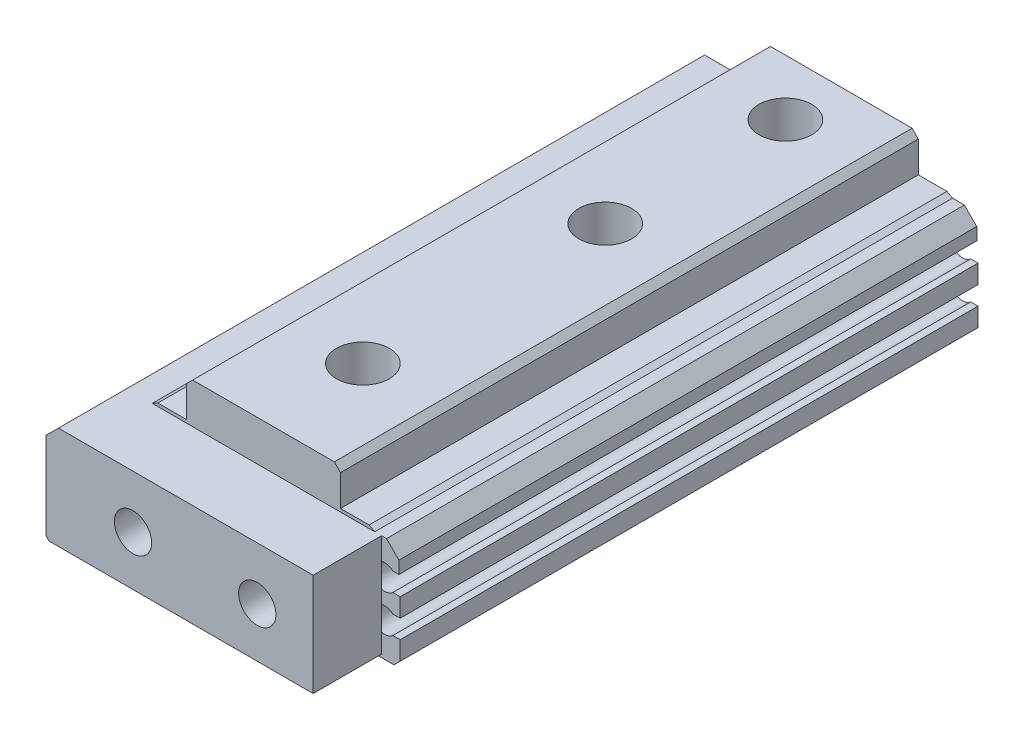
from build123d import *

# Parameters (mm, degrees)
EXTRUDE_1_DEPTH             = 93
EXTRUDE_2_DEPTH             = 11
CUT_EXTRUDE_1_DEPTH         = 93
PATTERN_LINEAR_1_COUNT      = 2
PATTERN_LINEAR_1_PITCH      = 6
CUT_EXTRUDE_2_DEPTH         = 93
CUT_EXTRUDE_3_DEPTH         = 93
PATTERN_LINEAR_2_COUNT      = 2
PATTERN_LINEAR_2_PITCH      = 8
PATTERN_LINEAR_2_COUNT_DIR2 = 2
PATTERN_LINEAR_2_PITCH_DIR2 = 20
PATTERN_LINEAR_3_COUNT      = 2
PATTERN_LINEAR_3_PITCH      = 20
CUT_EXTRUDE_4_DEPTH         = 4
PATTERN_LINEAR_4_COUNT      = 2
PATTERN_LINEAR_4_PITCH      = 58
SKETCH_16_W                 = 1
SKETCH_16_H                 = 9.5
CUT_EXTRUDE_5_DEPTH         = 46
SKETCH_21_W                 = 2
SKETCH_21_H                 = 4
CUT_EXTRUDE_6_DEPTH         = 93
PATTERN_LINEAR_5_COUNT      = 2
PATTERN_LINEAR_5_PITCH      = 8
HOLE_WIZARD_4_D             = 13
HOLE_WIZARD_4_DEPTH         = 1
HOLE_WIZARD_5_D             = 13
HOLE_WIZARD_5_DEPTH         = 1
HOLE_WIZARD_6_D             = 4.134
HOLE_WIZARD_6_DEPTH         = 5
HOLE_WIZARD_6_CSINK_D       = 5
HOLE_WIZARD_6_CSINK_ANGLE   = 90
HOLE_WIZARD_6_TIP           = 1.193383006


with BuildPart() as part:
    # 草图1 → 凸台-拉伸1 (new body)
    with BuildSketch(Plane.XY):
        Polygon((-24, 1.5), (-22.5, 0), (22, 0), (22, 17), (17.9, 17), (17, 17.5), (12.4, 17.5), (12.4, 22.5), (11.4, 23.5), (-11.4, 23.5), (-12.4, 22.5), (-12.4, 17.5), (-17, 17.5), (-17.9, 17), (-22, 17), (-24, 15), align=None)
    extrude(amount=EXTRUDE_1_DEPTH)

    # 草图2 → 凸台-拉伸2 (add)
    with BuildSketch(Plane.XY.offset(93)):
        Polygon((-24, 1), (-23.5, 0.5), (19, 0.5), (19, 17), (-22, 17), (-24, 15), align=None)
    extrude(amount=EXTRUDE_2_DEPTH)

    # 草图3 → 切除-拉伸1 (cut)
    with BuildSketch(Plane.XY):
        with BuildLine():
            Line((20.822875656, 4), (22, 4))
            Line((22, 4), (22, 7))
            Line((22, 7), (20.822875656, 7))
            ThreePointArc((20.822875656, 7), (17.5, 5.5), (20.822875656, 4))
        make_face()
    cut_extrude_1 = extrude(amount=CUT_EXTRUDE_1_DEPTH, mode=Mode.SUBTRACT)

    # 阵列(线性)1: 切除-拉伸1 ×2
    with Locations(*[(0, i * PATTERN_LINEAR_1_PITCH, 0) for i in range(1, PATTERN_LINEAR_1_COUNT)]):
        add(cut_extrude_1, mode=Mode.SUBTRACT)

    # 草图5 → 切除-拉伸2 (cut)
    with BuildSketch(Plane.XY):
        with BuildLine():
            Line((4.7, 0), (16, 0))
            Line((16, 0), (14.927664784, 1.072335216))
            ThreePointArc((14.927664784, 1.072335216), (14.37434682, 1.353332174), (13.761801698, 1.253790561))
            ThreePointArc((13.761801698, 1.253790561), (10.233759649, 0.343332602), (6.659563577, 1.051242793))
            ThreePointArc((6.659563577, 1.051242793), (6.070298822, 1.121297778), (5.5450865, 0.8450865))
            Line((5.5450865, 0.8450865), (4.7, 0))
        make_face()
    extrude(amount=CUT_EXTRUDE_2_DEPTH, mode=Mode.SUBTRACT)

    # 草图6 → 切除-拉伸3 (cut)
    with BuildSketch(Plane.XY):
        with BuildLine():
            Line((-16, 0), (-4.7, 0))
            Line((-4.7, 0), (-5.5450865, 0.8450865))
            ThreePointArc((-5.5450865, 0.8450865), (-6.070298822, 1.121297778), (-6.659563577, 1.051242793))
            ThreePointArc((-6.659563577, 1.051242793), (-10.233759649, 0.343332602), (-13.761801698, 1.253790561))
            ThreePointArc((-13.761801698, 1.253790561), (-14.37434682, 1.353332174), (-14.927664784, 1.072335216))
            Line((-14.927664784, 1.072335216), (-16, 0))
        make_face()
    extrude(amount=CUT_EXTRUDE_3_DEPTH, mode=Mode.SUBTRACT)

    # 草图7 → 孔1 (revolve, cut)
    with BuildSketch(Plane(origin=(0, 4.5, 0), x_dir=(0, 1, 0), z_dir=(1, 0, 0))):
        Polygon((0, 0), (0, 6.935884786), (1.621, 6), (1.621, 0.379), (2, 0), align=None)
    hole_wizard_1 = revolve(axis=Axis((0, 4.5, -14.308894879), (0, 0, 1)), mode=Mode.SUBTRACT)

    # 阵列(线性)2: Hole Wizard 1 2 × 2
    with Locations(*[(-j * PATTERN_LINEAR_2_PITCH_DIR2, i * PATTERN_LINEAR_2_PITCH, 0) for i in range(PATTERN_LINEAR_2_COUNT) for j in range(PATTERN_LINEAR_2_COUNT_DIR2) if (i, j) != (0, 0)]):
        add(hole_wizard_1, mode=Mode.SUBTRACT)

    # 草图10 → 切除-旋转1 (revolve, cut)
    with BuildSketch(Plane(origin=(10, 0, 0), x_dir=(0, 0, -1), z_dir=(1, 0, 0)), mode=Mode.PRIVATE) as cut_revolve_1_sk:
        Polygon((-104, 8.5), (-104, 11.5), (-66.5, 11.5), (-66.5, 14.5), (-21.5, 14.5), (-21.5, 8.5), align=None)
    cut_revolve_1 = revolve(cut_revolve_1_sk.sketch.rotate(Axis((10, 8.5, 21.5), (0, 0, 1)), 270), axis=Axis((10, 8.5, 21.5), (0, 0, 1)), mode=Mode.SUBTRACT)

    # 阵列(线性)3: 切除-旋转1 ×2
    with Locations(*[(-i * PATTERN_LINEAR_3_PITCH, 0, 0) for i in range(1, PATTERN_LINEAR_3_COUNT)]):
        add(cut_revolve_1, mode=Mode.SUBTRACT)

    # 草图12 → 切除-拉伸4 (cut)
    with BuildSketch(Plane(origin=(0, 0, 0), x_dir=(1, 0, 0), z_dir=(0, 1, 0))):
        with BuildLine():
            Line((-21, -37.5), (-21, -38.5))
            ThreePointArc((-21, -38.5), (-19, -40.5), (-17, -38.5))
            Line((-17, -38.5), (-17, -37.5))
            ThreePointArc((-17, -37.5), (-19, -35.5), (-21, -37.5))
        make_face()
    extrude(amount=CUT_EXTRUDE_4_DEPTH, mode=Mode.SUBTRACT)

    # 草图13 → 孔2 (revolve, cut)
    with BuildSketch(Plane(origin=(-24, 8.5, 15), x_dir=(0, 0, 1), z_dir=(0, 1, 0))):
        Polygon((0, 0), (0, 6.193383006), (2.067, 5), (2.067, 0.433), (2.5, 0), align=None)
    hole_wizard_2 = revolve(axis=Axis((-38.308894879, 8.5, 15), (1, 0, 0)), mode=Mode.SUBTRACT)

    # 阵列(线性)4: 孔2 ×2
    with Locations(*[(0, 0, i * PATTERN_LINEAR_4_PITCH) for i in range(1, PATTERN_LINEAR_4_COUNT)]):
        add(hole_wizard_2, mode=Mode.SUBTRACT)

    # 草图16 → 切除-拉伸5 (cut)
    with BuildSketch(Plane(origin=(0, 0, 0), x_dir=(1, 0, 0), z_dir=(0, 1, 0))):
        with Locations((-23.5, -86.25)):
            Rectangle(SKETCH_16_W, SKETCH_16_H)
    extrude(amount=CUT_EXTRUDE_5_DEPTH, mode=Mode.SUBTRACT)

    # 草图17 → 切除-旋转2 (revolve, cut)
    with BuildSketch(Plane.XY.offset(9), mode=Mode.PRIVATE) as cut_revolve_2_sk:
        Polygon((0, 23.5), (4.25, 23.5), (4.25, 16), (2.067, 16), (2.067, 0.433), (2.5, 0), (0, 0), align=None)
    revolve(cut_revolve_2_sk.sketch.rotate(Axis((0, 0, 9), (0, 1, 0)), 270), axis=Axis((0, 0, 9), (0, 1, 0)), mode=Mode.SUBTRACT)

    # 草图19 → 切除-旋转3 (revolve, cut)
    with BuildSketch(Plane.XY.offset(77), mode=Mode.PRIVATE) as cut_revolve_3_sk:
        Polygon((0, 23.5), (4.25, 23.5), (4.25, 16), (2.067, 16), (2.067, 0.433), (2.5, 0), (0, 0), align=None)
    revolve(cut_revolve_3_sk.sketch.rotate(Axis((0, 0, 77), (0, 1, 0)), 270), axis=Axis((0, 0, 77), (0, 1, 0)), mode=Mode.SUBTRACT)

    # 草图20 → 切除-旋转4 (revolve, cut)
    with BuildSketch(Plane.XY.offset(38), mode=Mode.PRIVATE) as cut_revolve_4_sk:
        Polygon((0, 23.5), (4.25, 23.5), (4.25, 16), (2.067, 16), (2.067, 0.433), (2.5, 0), (0, 0), align=None)
    revolve(cut_revolve_4_sk.sketch.rotate(Axis((0, 0, 38), (0, 1, 0)), 270), axis=Axis((0, 0, 38), (0, 1, 0)), mode=Mode.SUBTRACT)

    # 草图21 → 切除-旋转5 (revolve, cut)
    with BuildSketch(Plane.XY.offset(77), mode=Mode.PRIVATE) as cut_revolve_5_sk:
        with Locations((-20, 2)):
            Rectangle(SKETCH_21_W, SKETCH_21_H)
    revolve(cut_revolve_5_sk.sketch.rotate(Axis((-19, 4, 77), (0, -1, 0)), 90), axis=Axis((-19, 4, 77), (0, -1, 0)), mode=Mode.SUBTRACT)

    # 草图22 → 切除-拉伸6 (cut)
    with BuildSketch(Plane.XY):
        Polygon((19.8, 17), (21.8, 15), (21.8, 11.5), (22, 11.5), (22, 1), (21, 0), (24, 0), (24, 17), align=None)
    extrude(amount=CUT_EXTRUDE_6_DEPTH, mode=Mode.SUBTRACT)

    # 草图23 → 孔3 (revolve, cut)
    with BuildSketch(Plane(origin=(-23, 5, 86.25), x_dir=(0, 0, 1), z_dir=(0, 1, 0))):
        Polygon((0, 0), (0, 6.935884786), (1.621, 6), (1.621, 0.379), (2, 0), align=None)
    hole_wizard_3 = revolve(axis=Axis((-37.308894879, 5, 86.25), (1, 0, 0)), mode=Mode.SUBTRACT)

    # 阵列(线性)5: 孔3 ×2
    with Locations(*[(0, i * PATTERN_LINEAR_5_PITCH, 0) for i in range(1, PATTERN_LINEAR_5_COUNT)]):
        add(hole_wizard_3, mode=Mode.SUBTRACT)

    # 孔4
    with Locations(Plane(origin=(0, 0, 0), x_dir=(-1, 0, 0), z_dir=(0, 0, -1))):
        with Locations((-10, 8.5)):
            Hole(HOLE_WIZARD_4_D / 2, depth=HOLE_WIZARD_4_DEPTH)

    # 孔5
    with Locations(Plane(origin=(0, 0, 0), x_dir=(-1, 0, 0), z_dir=(0, 0, -1))):
        with Locations((10, 8.5)):
            Hole(HOLE_WIZARD_5_D / 2, depth=HOLE_WIZARD_5_DEPTH)

    # 孔6
    with Locations(Plane.ZY.offset(24)):
        with Locations((98.5, 10)):
            CounterSinkHole(HOLE_WIZARD_6_D / 2, HOLE_WIZARD_6_CSINK_D / 2, depth=HOLE_WIZARD_6_DEPTH, counter_sink_angle=HOLE_WIZARD_6_CSINK_ANGLE)
            with Locations((0, 0, -(HOLE_WIZARD_6_DEPTH + HOLE_WIZARD_6_TIP / 2))):  # 120° drill point
                Cone(0, HOLE_WIZARD_6_D / 2, HOLE_WIZARD_6_TIP, mode=Mode.SUBTRACT)


solid = part.part
